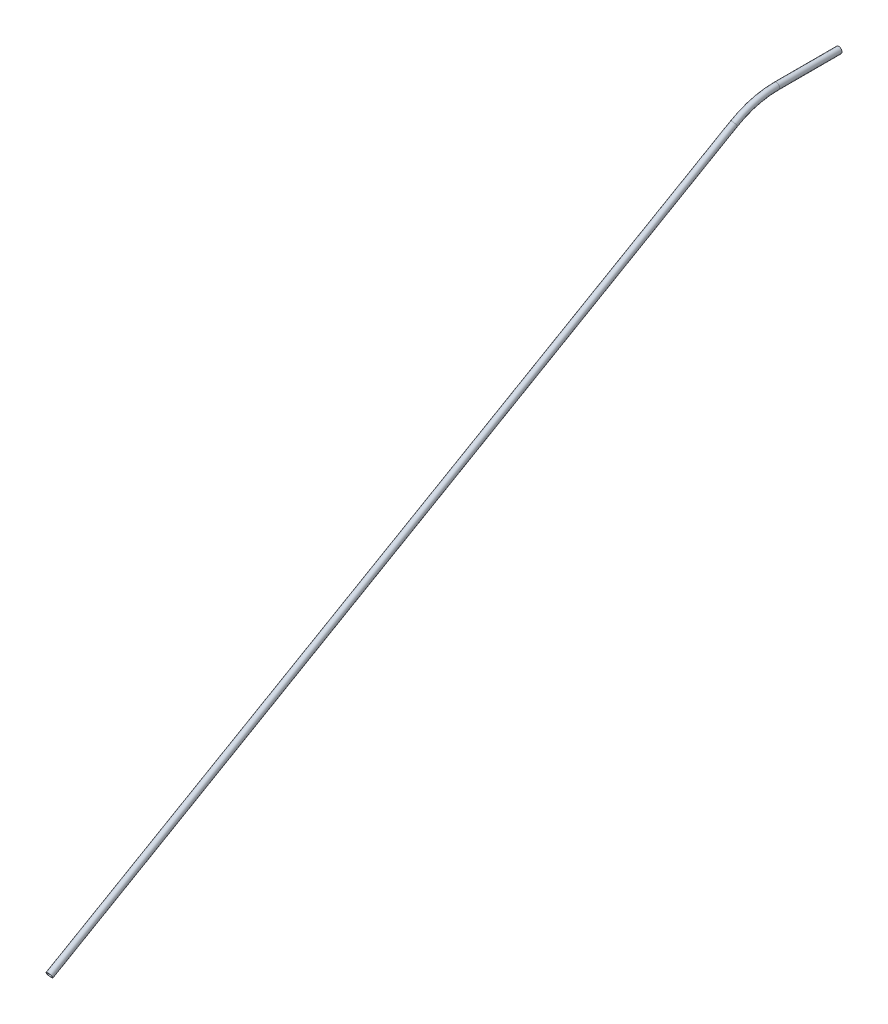
SolidWorks part; units mm, degrees
material "Q235"
ref_plane "Front Plane" through (0, 0, 0) normal (0, 0, 1) x (1, 0, 0)
ref_plane "Top Plane" through (0, 0, 0) normal (0, 1, 0) x (1, 0, 0)
ref_plane "Right Plane" through (0, 0, 0) normal (1, 0, 0) x (0, 0, -1)
sketch "Sketch1" plane through (0, 0, 0) normal (0, 0, 1) x (1, 0, 0)
  circle A0 centre (0, 0) radius 11
  circle A1 centre (0, 0) radius 9
  dimension "D1" = 2
  dimension "D2" = 22
sketch "Sketch2" plane through (0, 0, 0) normal (1, 0, 0) x (0, 0, -1)
  line L0 (0, 0) -> (-219.6152, 0)
  line L1 (-369.6152, -40.1924) -> (-2780.2968, -1432)
  arc A0 (-219.6152, 0) -> (-369.6152, -40.1924) centre (-219.6152, -300) ccw
  point P6 (-300, 0)
  dimension "D4" = 300
  dimension "D1" = 300
  dimension "D2" = 30
  dimension "D3" = 1432
sweep "Sweep1" add profiles "Sketch1" path "Sketch2"
